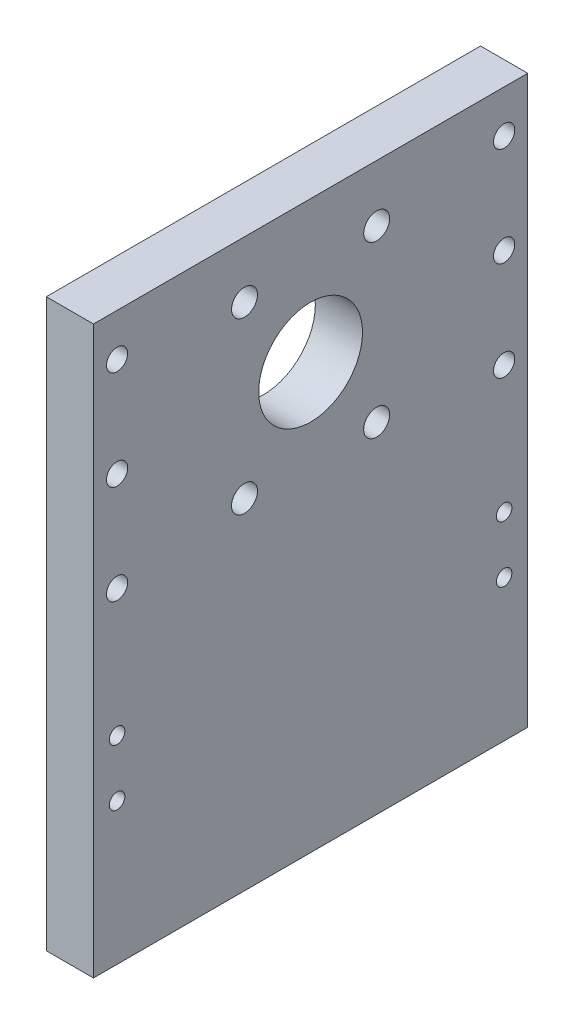
SolidWorks part; units mm, degrees
ref_plane "Front Plane" through (0, 0, 0) normal (0, 0, 1) x (1, 0, 0)
ref_plane "Top Plane" through (0, 0, 0) normal (0, 1, 0) x (1, 0, 0)
ref_plane "Right Plane" through (0, 0, 0) normal (1, 0, 0) x (0, 0, -1)
sketch "Sketch1" plane through (0, 0, 0) normal (1, 0, 0) x (0, 0, -1)
  line L1 (-46, 60) -> (46, 60)
  line L2 (-46, 60) -> (-46, -60)
  line L3 (-46, -60) -> (46, -60)
  line L4 (46, 60) -> (46, -60)
  line L5 (-46, 60) -> (46, -60) construction
  line L6 (-46, -60) -> (46, 60) construction
  point P0 (0, 0)
  dimension "D1" = 92
  dimension "D2" = 120
extrude "Boss-Extrude1" add sketch "Sketch1" along normal mid plane 10
sketch "Sketch2" plane through (5, 0, 0) normal (1, 0, 0) x (0, 0, -1)
  circle A0 centre (0, 30) radius 11
  dimension "D1" = 22
  dimension "D2" = 30
extrude "Cut-Extrude1" cut sketch "Sketch2" against normal through all
hole_wizard "M4 Tapped Hole1" positions "Sketch3" profile "Sketch4" tap size "M4" standard "ISO" end condition through all
sketch "Sketch3" plane through (5, 0, 0) normal (1, 0, 0) x (0, 0, -1)
  line L0 (-46, -60) -> (46, -60) construction
  line L1 (-46, 60) -> (-46, -60) construction
  line L2 (46, -60) -> (46, 60) construction
  point P0 (-41, -30)
  point P2 (-41, -18)
  point P4 (41, -30)
  point P6 (41, -18)
  dimension "D1" = 30
  dimension "D2" = 12
  dimension "D3" = 5
  dimension "D4" = 5
sketch "Sketch4" plane through (5, -30, 41) normal (0, 1, 0) x (0, 0, -1)
  line L0 (0, 0) -> (0, 10)
  line L1 (0, 10) -> (1.65, 10)
  line L2 (1.65, 10) -> (1.65, 0)
  line L5 (1.65, 0) -> (0, 0)
  line L11 (0, -6.35) -> (0, 107.95) construction
  dimension "通孔螺纹孔钻头直径" = 3.3
  dimension "通孔螺纹孔钻头深度" = 10
cosmetic thread "Cosmetic Thread1" parameters "D2"=4
cosmetic thread "Cosmetic Thread2" parameters "D2"=4
cosmetic thread "Cosmetic Thread3" parameters "D2"=4
cosmetic thread "Cosmetic Thread4" parameters "D2"=4
hole_wizard "CBORE for M4 Hex Socket Head Cap Screw1" positions "Sketch5" profile "Sketch6" counterbore size "M4" standard "ISO" end condition through all
sketch "Sketch5" plane through (-5, 0, 0) normal (-1, 0, 0) x (0, 0, 1)
  line L0 (-46, 60) -> (46, 60) construction
  line L1 (-46, -60) -> (-46, 60) construction
  line L2 (46, 60) -> (46, -60) construction
  point P0 (-41, 51)
  point P2 (-41, 30)
  point P4 (-41, 9)
  point P6 (41, 51)
  point P8 (41, 30)
  point P10 (41, 9)
  dimension "D1" = 9
  dimension "D2" = 21
  dimension "D3" = 21
  dimension "D4" = 5
  dimension "D5" = 5
sketch "Sketch6" plane through (-5, 51, -41) normal (0, 1, 0) x (0, 0, 1)
  line L0 (0, 0) -> (0, 10)
  line L1 (0, 10) -> (2.25, 10)
  line L3 (2.25, 10) -> (2.25, 4.4)
  line L4 (2.25, 4.4) -> (4, 4.4)
  line L5 (4, 4.4) -> (4, 0)
  line L7 (4, 0) -> (0, 0)
  line L11 (0, -6.35) -> (0, 107.95) construction
  dimension "通孔孔直径" = 4.5
  dimension "通孔孔深度" = 10
  dimension "柱形沉头孔直径" = 8
  dimension "柱形沉头孔深度" = 4.4
hole_wizard "CBORE for M5 Hex Socket Head Cap Screw1" positions "Sketch7" profile "Sketch8" counterbore size "M5" standard "ISO"
sketch "Sketch7" plane through (-5, 0, 0) normal (-1, 0, 0) x (0, 0, 1)
  line L0 (0, 30) -> (0, 98.2104) construction
  line L2 (0, 30) -> (27.7022, 30) construction
  point P0 (-14, 48)
  point P2 (14, 48)
  point P4 (-14, 12)
  point P6 (14, 12)
  dimension "D1" = 36
  dimension "D2" = 28
sketch "Sketch8" plane through (-5, 48, -14) normal (0, 1, 0) x (0, 0, 1)
  line L0 (0, 0) -> (0, 11.7524)
  line L1 (0, 11.7524) -> (2.75, 10.1)
  line L2 (2.75, 10.1) -> (2.75, 5.4)
  line L3 (2.75, 5.4) -> (5, 5.4)
  line L4 (5, 5.4) -> (5, 0)
  line L5 (5, 0) -> (0, 0)
  line L10 (0, 11.7524) -> (-2.75, 10.1) construction
  line L11 (0, -6.35) -> (0, 107.95) construction
  dimension "孔直径" = 5.5
  dimension "孔深度" = 10.1
  dimension "柱形沉头孔直径" = 10
  dimension "柱形沉头孔深度" = 5.4
  dimension "导头角度" = 118
